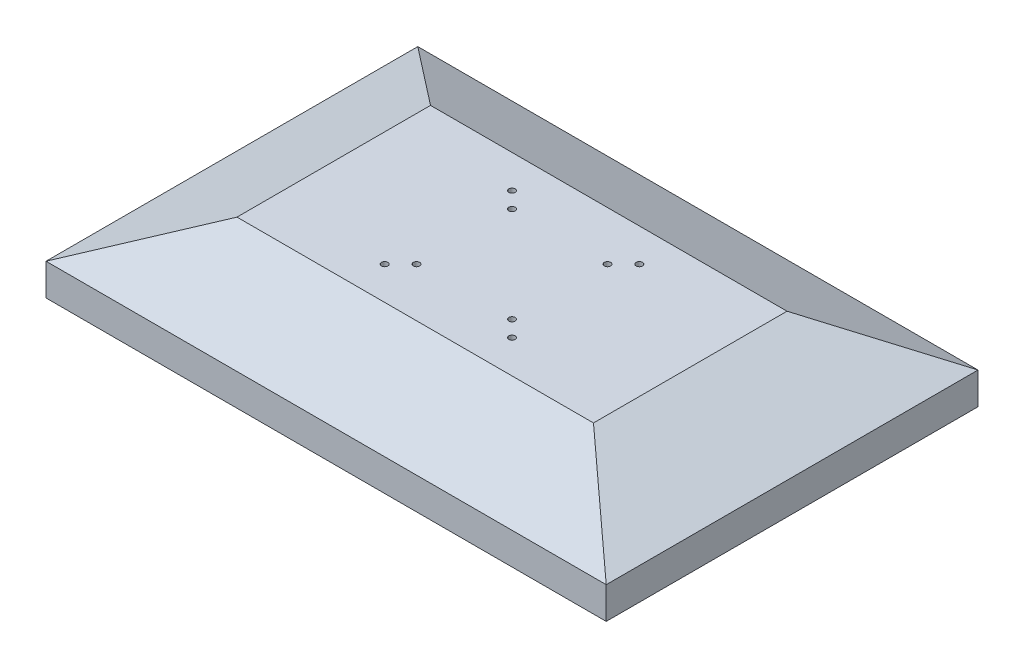
SolidWorks part; units mm, degrees
ref_plane "前视" through (0, 0, 0) normal (0, 0, 1) x (1, 0, 0)
ref_plane "上视" through (0, 0, 0) normal (0, 1, 0) x (1, 0, 0)
ref_plane "右视" through (0, 0, 0) normal (1, 0, 0) x (0, 0, -1)
sketch "草图1" plane through (0, 0, 0) normal (0, 1, 0) x (1, 0, 0)
  line L0 (0, 0) -> (0, 46.3441) construction
  line L1 (0, 0) -> (440, 0) construction
  line L3 (0, 0) -> (440, 0)
  line L4 (0, 0) -> (0, 292)
  line L5 (0, 292) -> (440, 292)
  line L6 (440, 0) -> (440, 292)
  dimension "D1" = 440
  dimension "D2" = 292
extrude "凸台-拉伸1" add sketch "草图1" along normal blind 60
sketch "草图3" plane through (0, 0, -292) normal (0, 0, -1) x (-1, 0, 0)
  line L0 (-440, 60) -> (-440, 25)
  line L1 (-440, 60) -> (-360, 60)
  line L2 (-440, 60) -> (0, 60) construction
  line L3 (-360, 60) -> (-440, 25)
  line L5 (-220, 0) -> (-220, 149.3803) construction
  line L6 (-440, 0) -> (0, 0) construction
  line L7 (-80, 60) -> (0, 25)
  line L8 (0, 60) -> (-80, 60)
  line L9 (0, 60) -> (0, 25)
extrude "切除-拉伸1" cut sketch "草图3" against normal blind 379
sketch "草图4" plane through (0, 0, 0) normal (-1, 0, 0) x (0, 0, 1)
  line L0 (-292, 60) -> (-292, 25)
  line L1 (-292, 60) -> (-222, 60)
  line L2 (-292, 60) -> (0, 60) construction
  line L3 (-222, 60) -> (-292, 25)
  line L4 (-146, 60) -> (-146, -16.2895) construction
  line L5 (-70, 60) -> (0, 25)
  line L6 (0, 60) -> (-70, 60)
  line L7 (0, 60) -> (0, 25)
extrude "切除-拉伸2" cut sketch "草图4" against normal blind 467
sketch "草图5" plane through (0, 60, 0) normal (0, 1, 0) x (1, 0, 0)
  line L0 (220, 222) -> (220, 21.1979) construction
  line L1 (360, 222) -> (80, 222) construction
  line L2 (0, 146) -> (407.3459, 146) construction
  line L4 (0, 0) -> (0, 292) construction
  line L7 (220, 146) -> (264.409, 190.409) construction
  circle A0 centre (270, 196) radius 2.5
  circle A1 centre (257.5, 183.5) radius 2.5
  circle A2 centre (270, 96) radius 2.5
  circle A3 centre (257.5, 108.5) radius 2.5
  circle A4 centre (170, 96) radius 2.5
  circle A5 centre (182.5, 108.5) radius 2.5
  circle A6 centre (170, 196) radius 2.5
  circle A7 centre (182.5, 183.5) radius 2.5
  dimension "D2" = 50
  dimension "D3" = 50
  dimension "D4" = 5
  dimension "D5" = 37.5
  dimension "D1" = 45
extrude "切除-拉伸3" cut sketch "草图5" against normal blind 20
